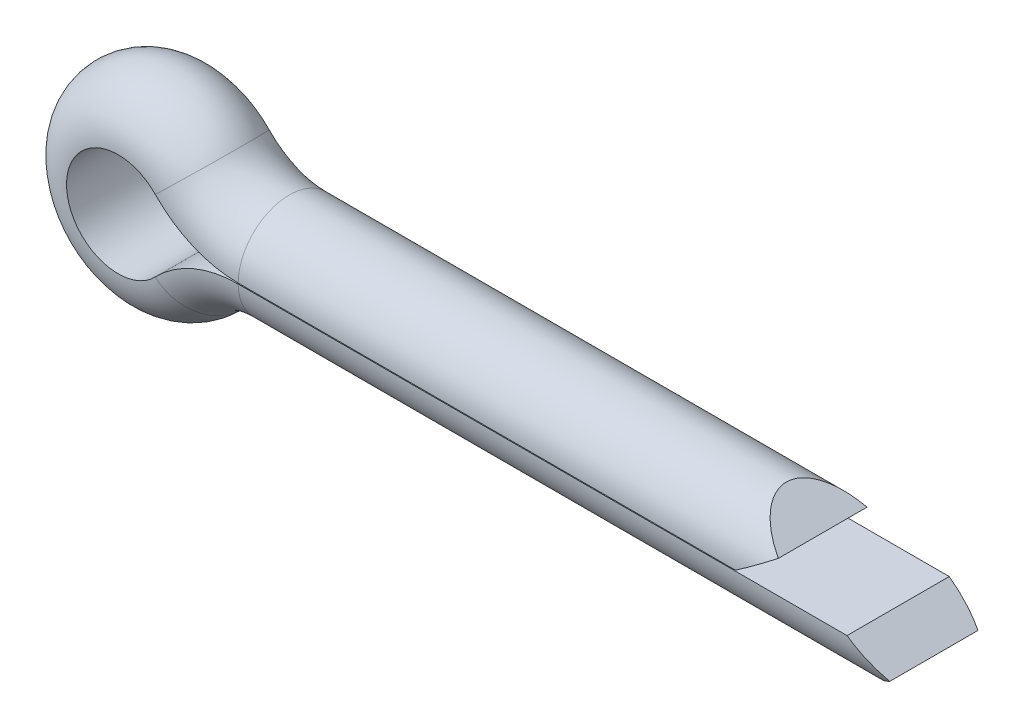
SolidWorks part; units mm, degrees
ref_plane "Front Plane" through (0, 0, 0) normal (0, 0, 1) x (1, 0, 0)
ref_plane "Top Plane" through (0, 0, 0) normal (0, 1, 0) x (1, 0, 0)
ref_plane "Right Plane" through (0, 0, 0) normal (1, 0, 0) x (0, 0, -1)
sketch "Dimension Sketch" plane through (0, 0, 0) normal (0, 0, 1) x (1, 0, 0)
  line L0 (14.7, 1.15) -> (2.7, 1.15)
  line L1 (2.7, -1.15) -> (17.2, -1.15)
  line L2 (2.7, 0) -> (27.3859, 0) construction
  line L3 (2.7, 0) -> (2.7, -0.0723) construction
  line L4 (-2.3, 0) -> (-2.3, 18.8979) construction
  arc A0 (2.7, 1.15) -> (1.6584, 1.5936) centre (2.7, 2.5946) cw
  arc A1 (1.6584, 1.5936) -> (1.6584, -1.5936) centre (0, 0) ccw
  arc A2 (1.6584, -1.5936) -> (2.7, -1.15) centre (2.7, -2.5946) cw
  dimension "c" = 4.6
  dimension "d1" = 2.3
  dimension "b" = 5
  dimension "l" = 12
  dimension "a" = 2.5
ref_plane "Plane1" through (14.7, 1.15, 0) normal (-1, 0, 0) x (0, 0, 1)
sketch "Sketch2" plane through (14.7, 1.15, 0) normal (-1, 0, 0) x (0, 0, 1)
  line L0 (0, -3.45) -> (0, 1.15) construction
  line L1 (-1.15, -1.14) -> (1.15, -1.14)
  arc A0 (1.15, -1.14) -> (-1.15, -1.14) centre (0, -1.15) ccw
  dimension "d" = 2.3
  dimension "D1" = 0.01
sweep "Sweep2" add profiles "Sketch2" path "Dimension Sketch"
sketch "Sketch3" plane through (0, 0, 0) normal (0, 0, 1) x (1, 0, 0)
  line L0 (2.7, 0) -> (2.7, 16.2682) construction
  line L1 (2.7, 0) -> (37.4999, 0) construction
  line L2 (17.2, -1.15) -> (17.2, -0.01) construction
  line L3 (14.7, 0.57) -> (13.8823, 1.15)
  line L4 (14.7, 1.15) -> (2.7, 1.15) construction
  line L5 (2.7, -1.15) -> (17.2, -1.15) construction
  line L6 (14.7, 0.57) -> (13.8753, 0)
  line L7 (17.2, -0.58) -> (16.3823, 0)
  line L9 (17.2, -0.58) -> (16.3753, -1.15)
  line L10 (16.3823, 0) -> (13.8753, 0)
  line L11 (13.8823, 1.15) -> (17.21, 1.15)
  line L12 (17.21, 1.15) -> (17.21, -1.15)
  line L13 (17.21, -1.15) -> (16.3753, -1.15)
  line L14 (14.7, 1.15) -> (14.7, 0.01) construction
  dimension "D1" = 0.01
  dimension "D3" = 70
  dimension "D4" = 70
extrude "Cut-Extrude1" cut sketch "Sketch3" against normal through all and the other way through all
